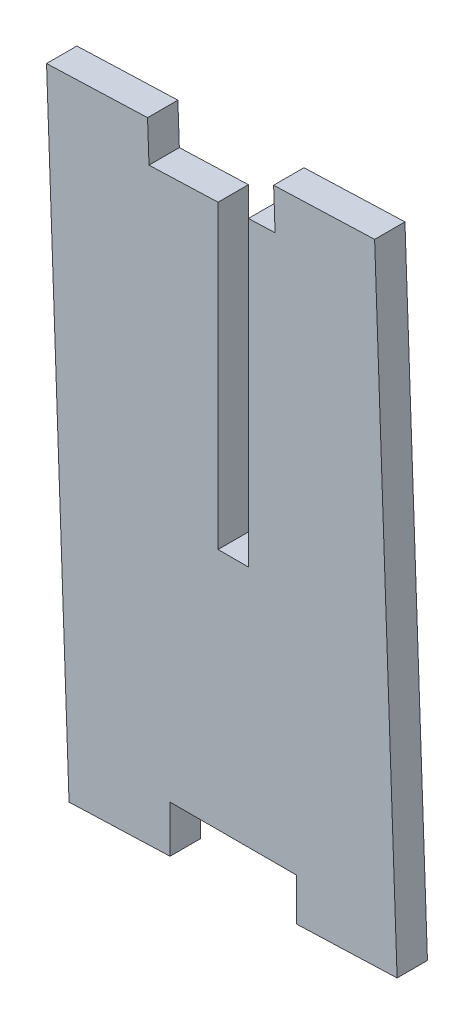
SolidWorks part; units mm, degrees
material "Q235B"
ref_plane "Front Plane" through (0, 0, 0) normal (0, 0, 1) x (1, 0, 0)
ref_plane "Top Plane" through (0, 0, 0) normal (0, 1, 0) x (1, 0, 0)
ref_plane "Right Plane" through (0, 0, 0) normal (1, 0, 0) x (0, 0, -1)
sketch "Sketch1" plane through (0, 0, 0) normal (0, 0, 1) x (1, 0, 0)
  line L0 (135.3194, 83.3626) -> (139.5206, -34.0083) construction
  line L1 (167.7656, 84.524) -> (98.1537, 84.524) construction
  line L2 (107.0364, -34.1088) -> (102.587, 90.1961)
  line L3 (107.0364, -34.1088) -> (127.0133, -33.3937)
  line L4 (127.0133, -33.3937) -> (127.0133, -24.1088)
  line L5 (152.014, -32.4988) -> (171.9288, -31.786)
  line L6 (122.85, 82.9163) -> (122.5638, 90.9112)
  line L7 (171.9288, -31.786) -> (167.4794, 92.5189)
  line L8 (147.7888, 83.809) -> (122.85, 82.9163)
  line L9 (127.0133, -24.1088) -> (152.014, -24.1088)
  line L10 (152.014, -24.1088) -> (152.014, -32.4988)
  line L11 (122.5638, 90.9112) -> (102.587, 90.1961)
  line L12 (147.7888, 83.809) -> (147.5026, 91.8038)
  line L13 (147.5026, 91.8038) -> (167.4794, 92.5189)
  dimension "D1" = 2.05
  dimension "D2" = 90
  dimension "D3" = 8
  dimension "D4" = 116.31
  dimension "D5" = 9.2849
  dimension "D7" = 90
extrude "Boss-Extrude1" add sketch "Sketch1" along normal blind 6
sketch "Sketch2" plane through (0, 0, 6) normal (0, 0, 1) x (1, 0, 0)
  line L0 (136.5136, 23.9104) -> (142.5136, 23.9104)
  line L2 (136.5136, 83.8856) -> (136.5136, 23.9104)
  line L3 (142.5136, 83.8856) -> (142.5136, 23.9104)
  line L4 (136.5136, 83.8856) -> (142.5136, 83.8856)
  line L8 (127.0133, -24.1088) -> (152.014, -24.1088) construction
  point P3 (139.5136, -24.1088)
  point P8 (139.5136, 23.9104)
  dimension "D1" = 6
extrude "Cut-Extrude1" cut sketch "Sketch2" against normal blind 6
